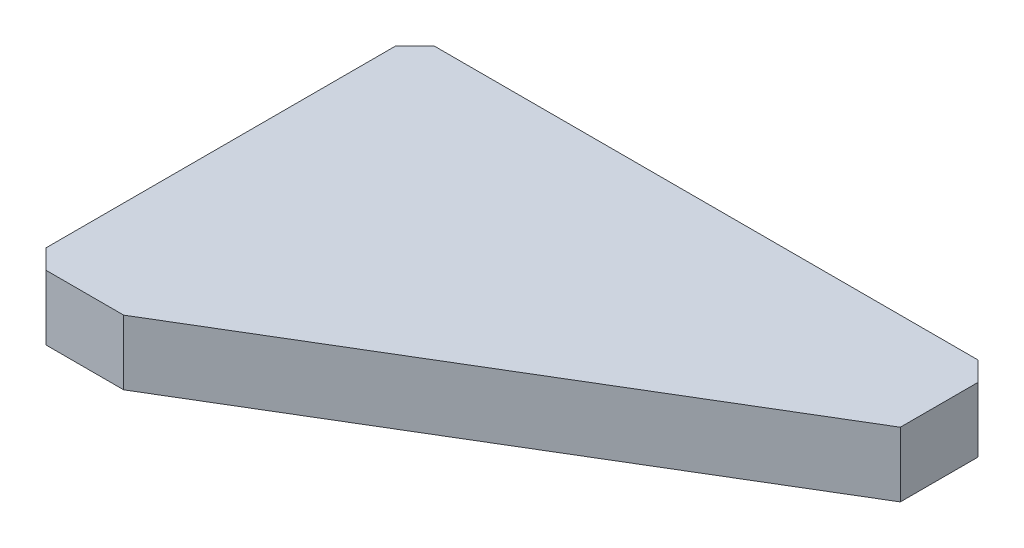
from build123d import *

# Parameters (mm, degrees)
SKETCH_1_W             = 90
SKETCH_1_H             = 60
EXTRUDE_1_DEPTH        = 10
CUT_EXTRUDE_1_DEPTH    = 15
CHAMFER_1_SIZE         = 3
HOLE_WIZARD_M5_1_D     = 4.2
HOLE_WIZARD_M5_1_DEPTH = 12.4
HOLE_WIZARD_M5_1_TIP   = 1.2618073
HOLE_WIZARD_M5_2_D     = 4.2
HOLE_WIZARD_M5_2_DEPTH = 12.4
HOLE_WIZARD_M5_2_TIP   = 1.2618073


with BuildPart() as part:
    # 草图1 → 凸台-拉伸1 (new body)
    with BuildSketch(Plane(origin=(0, 0, 0), x_dir=(1, 0, 0), z_dir=(0, 1, 0))):
        Rectangle(SKETCH_1_W, SKETCH_1_H)
    extrude(amount=EXTRUDE_1_DEPTH)

    # 草图2 → 切除-拉伸1 (cut)
    with BuildSketch(Plane(origin=(0, 10, 0), x_dir=(1, 0, 0), z_dir=(0, 1, 0))):
        Polygon((45, 15), (-30, -30), (45, -30), align=None)
    extrude(amount=-CUT_EXTRUDE_1_DEPTH, mode=Mode.SUBTRACT)

    # 倒角1
    chamfer_1_edges = [part.edges().sort_by_distance(p)[0] for p in [
        (-45, 5, 30),
        (-45, 5, -30),
        (45, 5, -30),
    ]]
    chamfer(chamfer_1_edges, length=CHAMFER_1_SIZE)

    # M5 螺纹孔1
    with Locations(Plane.ZY.offset(45)):
        with Locations((-15, 5), (15, 5)):
            Hole(HOLE_WIZARD_M5_1_D / 2, depth=HOLE_WIZARD_M5_1_DEPTH)
            with Locations((0, 0, -(HOLE_WIZARD_M5_1_DEPTH + HOLE_WIZARD_M5_1_TIP / 2))):  # 118° drill point
                Cone(0, HOLE_WIZARD_M5_1_D / 2, HOLE_WIZARD_M5_1_TIP, mode=Mode.SUBTRACT)

    # M5 螺纹孔2
    with Locations(Plane(origin=(0, 0, -30), x_dir=(-1, 0, 0), z_dir=(0, 0, -1))):
        with Locations((30, 5), (0, 5), (-30, 5)):
            Hole(HOLE_WIZARD_M5_2_D / 2, depth=HOLE_WIZARD_M5_2_DEPTH)
            with Locations((0, 0, -(HOLE_WIZARD_M5_2_DEPTH + HOLE_WIZARD_M5_2_TIP / 2))):  # 118° drill point
                Cone(0, HOLE_WIZARD_M5_2_D / 2, HOLE_WIZARD_M5_2_TIP, mode=Mode.SUBTRACT)


solid = part.part
